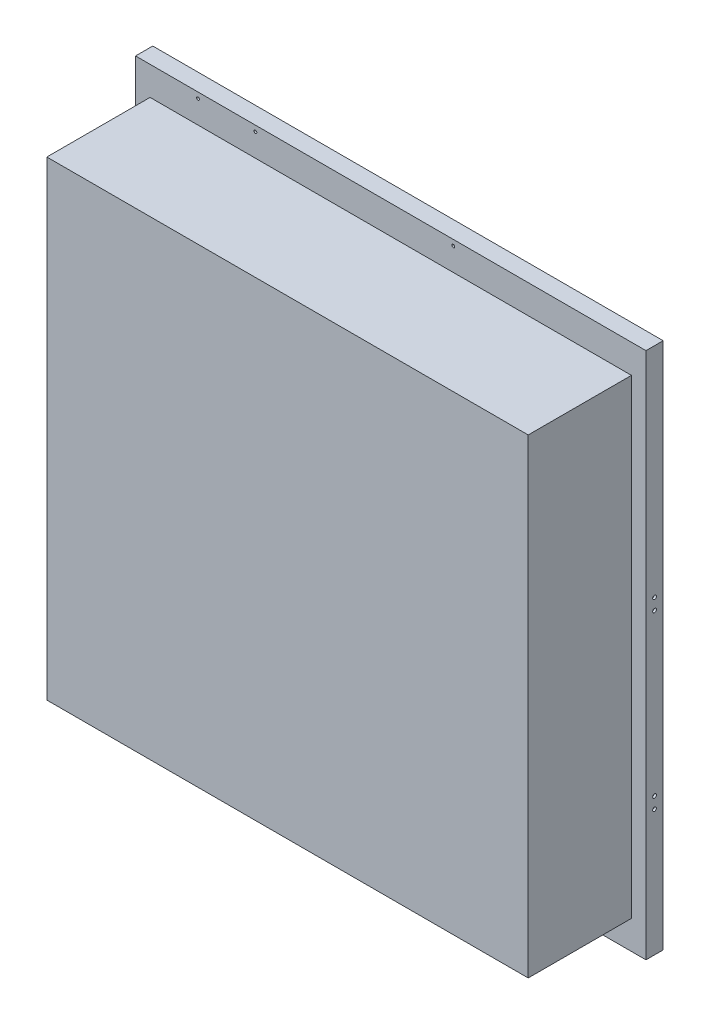
SolidWorks part; units mm, degrees
material "渡锌板"
ref_plane "前视基准面" through (0, 0, 0) normal (0, 0, 1) x (1, 0, 0)
ref_plane "上视基准面" through (0, 0, 0) normal (0, 1, 0) x (1, 0, 0)
ref_plane "右视基准面" through (0, 0, 0) normal (1, 0, 0) x (0, 0, -1)
sketch "草图1" plane through (0, 0, 0) normal (0, 0, 1) x (1, 0, 0)
  line L1 (-222.5, -235) -> (222.5, -235)
  line L2 (-222.5, -235) -> (-222.5, 235)
  line L3 (-222.5, 235) -> (222.5, 235)
  line L4 (222.5, -235) -> (222.5, 235)
  line L5 (-222.5, -235) -> (222.5, 235) construction
  line L6 (-222.5, 235) -> (222.5, -235) construction
  point P0 (0, 0)
  dimension "D1" = 445
  dimension "D2" = 470
extrude "凸台-拉伸1" add sketch "草图1" along normal mid plane 15
shell "抽壳1" thickness 2
sketch "草图2" plane through (0, 0, -7.5) normal (0, 0, -1) x (-1, 0, 0)
  line L0 (222.5, 235) -> (222.5, -235) construction
  line L1 (-212.5, -225) -> (212.5, -225)
  line L2 (-212.5, -225) -> (-212.5, 225)
  line L3 (-212.5, 225) -> (212.5, 225)
  line L4 (212.5, -225) -> (212.5, 225)
  line L5 (-212.5, -225) -> (212.5, 225) construction
  line L6 (-212.5, 225) -> (212.5, -225) construction
  line L7 (-222.5, 235) -> (222.5, 235) construction
  point P0 (0, 0)
  dimension "D1" = 10
  dimension "D2" = 10
extrude "切除-拉伸1" cut sketch "草图2" against normal blind 2
sketch "草图3" plane through (0, 0, 7.5) normal (0, 0, 1) x (1, 0, 0)
  line L0 (-205, 150) -> (-195, 150) construction
  line L1 (-200, -150) -> (200, -150) construction
  line L2 (-200, -150) -> (-200, 150) construction
  line L3 (-200, 150) -> (200, 150) construction
  line L4 (200, -150) -> (200, 150) construction
  line L5 (-200, -150) -> (200, 150) construction
  line L6 (-200, 150) -> (200, -150) construction
  line L7 (-205, 152.5) -> (-195, 152.5)
  line L8 (-205, 147.5) -> (-195, 147.5)
  line L9 (0, 235) -> (0, -235) construction
  line L10 (222.5, 235) -> (-222.5, 235) construction
  line L11 (-222.5, -235) -> (222.5, -235) construction
  line L12 (-222.5, 0) -> (222.5, 0) construction
  line L13 (-222.5, 235) -> (-222.5, -235) construction
  line L14 (222.5, -235) -> (222.5, 235) construction
  line L15 (195, 150) -> (205, 150) construction
  line L16 (195, 152.5) -> (205, 152.5)
  line L17 (195, 147.5) -> (205, 147.5)
  line L18 (-205, -150) -> (-195, -150) construction
  line L19 (-205, -147.5) -> (-195, -147.5)
  line L20 (-205, -152.5) -> (-195, -152.5)
  line L21 (195, -150) -> (205, -150) construction
  line L22 (195, -147.5) -> (205, -147.5)
  line L23 (195, -152.5) -> (205, -152.5)
  arc A0 (-205, 152.5) -> (-205, 147.5) centre (-205, 150) ccw
  arc A1 (-195, 147.5) -> (-195, 152.5) centre (-195, 150) ccw
  arc A2 (195, 152.5) -> (195, 147.5) centre (195, 150) ccw
  arc A3 (205, 147.5) -> (205, 152.5) centre (205, 150) ccw
  arc A4 (-205, -147.5) -> (-205, -152.5) centre (-205, -150) ccw
  arc A5 (-195, -152.5) -> (-195, -147.5) centre (-195, -150) ccw
  arc A6 (195, -147.5) -> (195, -152.5) centre (195, -150) ccw
  arc A7 (205, -152.5) -> (205, -147.5) centre (205, -150) ccw
  point P0 (0, 0)
  point P8 (-200, 150)
  point P27 (200, 150)
  point P34 (-200, -150)
  point P41 (200, -150)
  dimension "D4" = 2.5
  dimension "D6" = 2.5
  dimension "D8" = 2.5
  dimension "D9" = 2.5
  dimension "D1" = 400
  dimension "D2" = 300
  dimension "D3" = 10
  dimension "D5" = 10
  dimension "D7" = 10
  dimension "D10" = 10
extrude "切除-拉伸2" cut sketch "草图3" against normal blind 10
sketch "草图4" plane through (0, 0, 7.5) normal (0, 0, 1) x (1, 0, 0)
  line L0 (-222.5, -235) -> (222.5, -235) construction
  line L2 (222.5, -235) -> (222.5, 235) construction
  line B0 (147.5, -212.75) -> (147.5, -217.25) construction
  line B1 (37.5, -212.75) -> (37.5, -217.25) construction
  line B2 (-72.5, -212.75) -> (-72.5, -217.25) construction
  line B3 (164.75, 68) -> (159.2455, 68) construction
  line B4 (164.75, -25) -> (159.4595, -25) construction
  line B5 (147.5, -62.75) -> (147.5, -67.25) construction
  line B6 (37.5, -62.75) -> (37.5, -67.25) construction
  line B7 (-72.5, -62.75) -> (-72.5, -67.25) construction
  line B8 (-180.25, -65) -> (-184.75, -65) construction
  line B9 (-182.5, -62.75) -> (-182.5, -67.25) construction
  line B10 (17.25, -24) -> (11.5, -24) construction
  line B11 (15, -21.75) -> (15, -26.25) construction
  line B12 (-86.5, -21.75) -> (-86.5, -26.25) construction
  line B13 (1.75, 168.5) -> (-2.75, 168.5) construction
  line B14 (-0.5, 170.75) -> (-0.5, 166.25) construction
  line B15 (102.75, 129) -> (98.25, 129) construction
  line B16 (100.5, 131.25) -> (100.5, 126.75) construction
  line B17 (56.75, 225) -> (52.25, 225) construction
  line B18 (56.75, 177) -> (52.25, 177) construction
  line B19 (-172.5, -212.75) -> (-172.5, -217.25) construction
  line B20 (195.25, 72.4966) -> (190.75, 72.4966) construction
  line B21 (195.25, -202.5) -> (190.75, -202.5) construction
  line B22 (195.25, -92.5) -> (190.75, -92.5) construction
  line B23 (195.25, 17.5) -> (190.75, 17.5) construction
  line B24 (195.25, 7.5) -> (190.75, 7.5) construction
  line B25 (195.25, 202.4966) -> (190.75, 202.4966) construction
  line B26 (-175.75, 225) -> (-180.25, 225) construction
  line B27 (-83, -24) -> (-88.9344, -24) construction
  line B28 (47.25, -22.5) -> (51.75, -22.5) construction
  line B29 (47.25, 70.5) -> (51.75, 70.5) construction
  line B30 (222.5, -235) -> (-227.5, -235) construction
  line B31 (-227.5, -235) -> (-227.5, 235) construction
  line B32 (-227.5, 235) -> (222.5, 235) construction
  line B33 (222.5, 235) -> (222.5, -235) construction
  line B34 (-200, -152.5) -> (-205, -152.5) construction
  line B35 (-205, -147.5) -> (-200, -147.5) construction
  line B36 (200, 147.5) -> (195, 147.5) construction
  line B37 (195, 152.5) -> (200, 152.5) construction
  line B38 (200, -152.5) -> (195, -152.5) construction
  line B39 (195, -147.5) -> (200, -147.5) construction
  line B40 (-200, 147.5) -> (-205, 147.5) construction
  line B41 (-205, 152.5) -> (-200, 152.5) construction
  line B42 (145.25, -103.5) -> (149.75, -103.5) construction
  line B43 (145.25, -166.5) -> (149.75, -166.5) construction
  line B44 (71.5, -132.75) -> (71.5, -137.25) construction
  line B45 (-88.5, -132.75) -> (-88.5, -137.25) construction
  line B46 (-86.25, -135) -> (-90.75, -135) construction
  line B47 (-168.5, -132.75) -> (-168.5, -137.25) construction
  line B48 (-43.5, -132.75) -> (-43.5, -137.25) construction
  line B49 (-41.25, -135) -> (-45.75, -135) construction
  arc B50 (152.5, 186.5) -> (154, 185) centre (152.5, 185) ccw
  circle B51 centre (152.5, 185) radius 1.3
  arc B52 (152.5, 88.5) -> (154, 87) centre (152.5, 87) ccw
  circle B53 centre (152.5, 87) radius 1.3
  arc B54 (147.5, -213.5) -> (149, -215) centre (147.5, -215) ccw
  circle B55 centre (147.5, -215) radius 1.3
  arc B56 (37.5, -213.5) -> (39, -215) centre (37.5, -215) ccw
  circle B57 centre (37.5, -215) radius 1.3
  arc B58 (-72.5, -213.5) -> (-71, -215) centre (-72.5, -215) ccw
  circle B59 centre (-72.5, -215) radius 1.3
  arc B60 (162.5, 69.5) -> (164, 68) centre (162.5, 68) ccw
  circle B61 centre (162.5, 68) radius 1.3
  arc B62 (162.5, -23.5) -> (164, -25) centre (162.5, -25) ccw
  circle B63 centre (162.5, -25) radius 1.3
  arc B64 (147.5, -63.5) -> (149, -65) centre (147.5, -65) ccw
  circle B65 centre (147.5, -65) radius 1.3
  arc B66 (37.5, -63.5) -> (39, -65) centre (37.5, -65) ccw
  circle B67 centre (37.5, -65) radius 1.3
  arc B68 (-72.5, -63.5) -> (-71, -65) centre (-72.5, -65) ccw
  circle B69 centre (-72.5, -65) radius 1.3
  arc B70 (-182.5, -63.5) -> (-181, -65) centre (-182.5, -65) ccw
  circle B71 centre (-182.5, -65) radius 1.3
  arc B72 (15, -22.5) -> (16.5, -24) centre (15, -24) ccw
  circle B73 centre (15, -24) radius 1.3
  arc B74 (-86.5, -22.5) -> (-85, -24) centre (-86.5, -24) ccw
  circle B75 centre (-86.5, -24) radius 1.3
  arc B76 (-0.5, 170) -> (1, 168.5) centre (-0.5, 168.5) ccw
  circle B77 centre (-0.5, 168.5) radius 1.3
  arc B78 (100.5, 130.5) -> (102, 129) centre (100.5, 129) ccw
  circle B79 centre (100.5, 129) radius 1.3
  arc B80 (-178, -13.5) -> (-176.5, -15) centre (-178, -15) ccw
  circle B81 centre (-178, -15) radius 1.3
  arc B82 (-128, -13.5) -> (-126.5, -15) centre (-128, -15) ccw
  circle B83 centre (-128, -15) radius 1.3
  arc B84 (54.5, 226.5) -> (56, 225) centre (54.5, 225) ccw
  circle B85 centre (54.5, 225) radius 1.3
  arc B86 (54.5, 178.5) -> (56, 177) centre (54.5, 177) ccw
  circle B87 centre (54.5, 177) radius 1.3
  arc B88 (-172.5, -213.5) -> (-171, -215) centre (-172.5, -215) ccw
  circle B89 centre (-172.5, -215) radius 1.3
  arc B90 (193, 73.9966) -> (194.5, 72.4966) centre (193, 72.4966) ccw
  circle B91 centre (193, 72.4966) radius 1.3
  arc B92 (193, -201) -> (194.5, -202.5) centre (193, -202.5) ccw
  circle B93 centre (193, -202.5) radius 1.3
  arc B94 (193, -91) -> (194.5, -92.5) centre (193, -92.5) ccw
  circle B95 centre (193, -92.5) radius 1.3
  arc B96 (193, 19) -> (194.5, 17.5) centre (193, 17.5) ccw
  circle B97 centre (193, 17.5) radius 1.3
  arc B98 (194.5, 7.5) -> (193, 6) centre (193, 7.5) ccw
  circle B99 centre (193, 7.5) radius 1.3
  arc B100 (193, 203.9966) -> (194.5, 202.4966) centre (193, 202.4966) ccw
  circle B101 centre (193, 202.4966) radius 1.3
  arc B102 (-178, 226.5) -> (-176.5, 225) centre (-178, 225) ccw
  circle B103 centre (-178, 225) radius 1.3
  arc B104 (-128, 226.5) -> (-126.5, 225) centre (-128, 225) ccw
  circle B105 centre (-128, 225) radius 1.3
  arc B106 (134.5, 186.5) -> (136, 185) centre (134.5, 185) ccw
  circle B107 centre (134.5, 185) radius 1.3
  arc B108 (134.5, 88.5) -> (136, 87) centre (134.5, 87) ccw
  circle B109 centre (134.5, 87) radius 1.3
  arc B110 (48, -22.5) -> (49.5, -21) centre (49.5, -22.5) ccw
  circle B111 centre (49.5, -22.5) radius 1.3
  arc B112 (48, 70.5) -> (49.5, 72) centre (49.5, 70.5) ccw
  circle B113 centre (49.5, 70.5) radius 1.3
  arc B114 (-205, -147.5) -> (-205, -152.5) centre (-205, -150) ccw construction
  arc B115 (-200, -152.5) -> (-200, -147.5) centre (-200, -150) ccw construction
  arc B116 (195, 152.5) -> (195, 147.5) centre (195, 150) ccw construction
  arc B117 (200, 147.5) -> (200, 152.5) centre (200, 150) ccw construction
  arc B118 (195, -147.5) -> (195, -152.5) centre (195, -150) ccw construction
  arc B119 (200, -152.5) -> (200, -147.5) centre (200, -150) ccw construction
  arc B120 (-205, 152.5) -> (-205, 147.5) centre (-205, 150) ccw construction
  arc B121 (-200, 147.5) -> (-200, 152.5) centre (-200, 150) ccw construction
  arc B122 (146, -103.5) -> (147.5, -102) centre (147.5, -103.5) ccw
  circle B123 centre (147.5, -103.5) radius 1.3
  arc B124 (146, -166.5) -> (147.5, -165) centre (147.5, -166.5) ccw
  circle B125 centre (147.5, -166.5) radius 1.3
  arc B126 (71.5, -133.5) -> (73, -135) centre (71.5, -135) ccw
  circle B127 centre (71.5, -135) radius 1.3
  arc B128 (-88.5, -133.5) -> (-87, -135) centre (-88.5, -135) ccw
  circle B129 centre (-88.5, -135) radius 1.3
  arc B130 (-168.5, -133.5) -> (-167, -135) centre (-168.5, -135) ccw
  circle B131 centre (-168.5, -135) radius 1.3
  arc B132 (-43.5, -133.5) -> (-42, -135) centre (-43.5, -135) ccw
  circle B133 centre (-43.5, -135) radius 1.3
sketch_block_instance "块1-1"
sketch_block "块1" parameters "D1"=1.5
hole_wizard "M3 螺纹孔1" positions "草图6" profile "草图5" tap size "M3" standard "GB"
sketch "草图6" plane through (0, 0, 7.5) normal (0, 0, 1) x (1, 0, 0)
  line L0 (222.5, 235) -> (-222.5, 235) construction
  line L1 (222.5, -235) -> (222.5, 235) construction
  line L2 (-222.5, 235) -> (-222.5, -235) construction
  line L3 (-222.5, -235) -> (222.5, -235) construction
  line L4 (-222.5, 235) -> (-222.5, -235) construction
  point P1 (-72.5, -215)
  point P4 (-172.5, -215)
  point P7 (37.5, -215)
  point P10 (147.5, -215)
  point P13 (193, -202.5)
  point P16 (147.5, -166.5)
  point P19 (66.5, -135)
  point P22 (-13.5, -135)
  point P25 (-58.5, -135)
  point P28 (-173.5, -135)
  point P31 (-182.5, -65)
  point P34 (-168, -15)
  point P37 (-118, -15)
  point P40 (-72.5, -65)
  point P43 (-81.5, -24)
  point P46 (37.5, -65)
  point P49 (15, -24)
  point P52 (49.5, -22.5)
  point P55 (147.5, -103.5)
  point P58 (193, -92.5)
  point P61 (147.5, -65)
  point P64 (162.5, -25)
  point P67 (193, 7.5)
  point P70 (193, 17.5)
  point P73 (193, 72.4966)
  point P76 (162.5, 68)
  point P79 (152.5, 27)
  point P82 (134.5, 27)
  point P85 (100.5, 129)
  point P88 (49.5, 70.5)
  point P91 (193, 202.4966)
  point P94 (152.5, 125)
  point P97 (134.5, 125)
  point P100 (54.5, 177)
  point P103 (54.5, 225)
  point P106 (4.5, 168.5)
  point P109 (-118, 225)
  point P112 (-168, 225)
  point P155 (-222.5, 0)
  dimension "D1" = 98
  dimension "D2" = 18
  dimension "D3" = 110
  dimension "D4" = 70
  dimension "D5" = 49
  dimension "D6" = 115
  dimension "D7" = 45
  dimension "D8" = 80
  dimension "D9" = 100
  dimension "D10" = 50
  dimension "D11" = 240
  dimension "D12" = 10
  dimension "D13" = 54.5
  dimension "D14" = 141
  dimension "D15" = 259
  dimension "D16" = 227
  dimension "D17" = 66.5
sketch "草图5" plane through (-72.5, -215, 7.5) normal (1, 0, 0) x (0, -1, 0)
  line L0 (0, 0) -> (0, 7.5)
  line L1 (0, 7.5) -> (1.25, 7.5)
  line L2 (1.25, 7.5) -> (1.25, 0)
  line L5 (1.25, 0) -> (0, 0)
  line L10 (0, 7.5) -> (-1.25, 7.5) construction
  line L11 (0, -6.35) -> (0, 107.95) construction
  dimension "螺纹孔钻头直径" = 2.5
  dimension "螺纹孔钻头深度" = 7.5
  dimension "导头角度" = 180
cosmetic thread "孔螺蚊线1" parameters "D1"=1.5, "D2"=3
cosmetic thread "孔螺蚊线2" parameters "D1"=1.5, "D2"=3
cosmetic thread "孔螺蚊线3" parameters "D1"=1.5, "D2"=3
cosmetic thread "孔螺蚊线4" parameters "D1"=1.5, "D2"=3
cosmetic thread "孔螺蚊线5" parameters "D1"=1.5, "D2"=3
cosmetic thread "孔螺蚊线6" parameters "D1"=1.5, "D2"=3
cosmetic thread "孔螺蚊线7" parameters "D1"=1.5, "D2"=3
cosmetic thread "孔螺蚊线8" parameters "D1"=1.5, "D2"=3
cosmetic thread "孔螺蚊线9" parameters "D1"=1.5, "D2"=3
cosmetic thread "孔螺蚊线10" parameters "D1"=1.5, "D2"=3
cosmetic thread "孔螺蚊线11" parameters "D1"=1.5, "D2"=3
cosmetic thread "孔螺蚊线12" parameters "D1"=1.5, "D2"=3
cosmetic thread "孔螺蚊线13" parameters "D1"=1.5, "D2"=3
cosmetic thread "孔螺蚊线14" parameters "D1"=1.5, "D2"=3
cosmetic thread "孔螺蚊线15" parameters "D1"=1.5, "D2"=3
cosmetic thread "孔螺蚊线16" parameters "D1"=1.5, "D2"=3
cosmetic thread "孔螺蚊线17" parameters "D1"=1.5, "D2"=3
cosmetic thread "孔螺蚊线18" parameters "D1"=1.5, "D2"=3
cosmetic thread "孔螺蚊线19" parameters "D1"=1.5, "D2"=3
cosmetic thread "孔螺蚊线20" parameters "D1"=1.5, "D2"=3
cosmetic thread "孔螺蚊线21" parameters "D1"=1.5, "D2"=3
cosmetic thread "孔螺蚊线22" parameters "D1"=1.5, "D2"=3
cosmetic thread "孔螺蚊线23" parameters "D1"=1.5, "D2"=3
cosmetic thread "孔螺蚊线24" parameters "D1"=1.5, "D2"=3
cosmetic thread "孔螺蚊线25" parameters "D1"=1.5, "D2"=3
cosmetic thread "孔螺蚊线26" parameters "D1"=1.5, "D2"=3
cosmetic thread "孔螺蚊线27" parameters "D1"=1.5, "D2"=3
cosmetic thread "孔螺蚊线28" parameters "D1"=1.5, "D2"=3
cosmetic thread "孔螺蚊线29" parameters "D1"=1.5, "D2"=3
cosmetic thread "孔螺蚊线30" parameters "D1"=1.5, "D2"=3
cosmetic thread "孔螺蚊线31" parameters "D1"=1.5, "D2"=3
cosmetic thread "孔螺蚊线32" parameters "D1"=1.5, "D2"=3
cosmetic thread "孔螺蚊线33" parameters "D1"=1.5, "D2"=3
cosmetic thread "孔螺蚊线34" parameters "D1"=1.5, "D2"=3
cosmetic thread "孔螺蚊线35" parameters "D1"=1.5, "D2"=3
cosmetic thread "孔螺蚊线36" parameters "D1"=1.5, "D2"=3
cosmetic thread "孔螺蚊线37" parameters "D1"=1.5, "D2"=3
cosmetic thread "孔螺蚊线38" parameters "D1"=1.5, "D2"=3
sketch "草图7" plane through (0, 235, 0) normal (0, 1, 0) x (1, 0, 0)
  line L0 (222.5, -7.5) -> (222.5, 7.5) construction
  line L1 (-222.5, 7.5) -> (222.5, 7.5)
  line L2 (-222.5, 7.5) -> (-222.5, -6)
  line L3 (-222.5, -6) -> (222.5, -6)
  line L4 (222.5, 7.5) -> (222.5, -6)
  line L5 (222.5, -7.5) -> (-222.5, -7.5) construction
  dimension "D1" = 1.5
extrude "切除-拉伸3" [suppressed] cut sketch "草图7" against normal through all
sketch "草图9" plane through (0, 0, 7.5) normal (0, 0, 1) x (1, 0, 0)
  line L0 (222.5, -235) -> (222.5, 235) construction
  line L1 (-222.5, 235) -> (222.5, 235)
  line L2 (-222.5, 235) -> (-222.5, 230)
  line L3 (-222.5, 230) -> (222.5, 230)
  line L4 (222.5, 235) -> (222.5, 230)
  line L6 (-222.5, -235) -> (222.5, -235)
  line L7 (-222.5, -235) -> (-222.5, -230)
  line L8 (-222.5, -230) -> (222.5, -230)
  line L9 (222.5, -235) -> (222.5, -230)
  dimension "D1" = 5
  dimension "D2" = 5
extrude "切除-拉伸4" cut sketch "草图9" against normal through all
sketch "草图10" plane through (0, 230, 0) normal (0, 1, 0) x (1, 0, 0)
  line L4 (-222.5, -7.5) -> (222.5, -7.5)
  line L5 (222.5, -7.5) -> (222.5, 7.5)
  line L6 (222.5, 7.5) -> (-222.5, 7.5)
  line L7 (-222.5, 7.5) -> (-222.5, -7.5)
  line L8 (-222.5, -7.5) -> (222.5, -7.5)
  line L9 (222.5, -7.5) -> (222.5, 7.5)
  line L10 (222.5, 7.5) -> (-222.5, 7.5)
  line L11 (-222.5, 7.5) -> (-222.5, -7.5)
  dimension "D1" = 0
extrude "凸台-拉伸2" add sketch "草图10" against normal blind 1.5
sketch "草图11" plane through (0, -230, 0) normal (0, -1, 0) x (1, 0, 0)
  line L4 (222.5, 7.5) -> (-222.5, 7.5)
  line L5 (-222.5, 7.5) -> (-222.5, -7.5)
  line L6 (-222.5, -7.5) -> (222.5, -7.5)
  line L7 (222.5, -7.5) -> (222.5, 7.5)
  line L8 (222.5, 7.5) -> (-222.5, 7.5)
  line L9 (-222.5, 7.5) -> (-222.5, -7.5)
  line L10 (-222.5, -7.5) -> (222.5, -7.5)
  line L11 (222.5, -7.5) -> (222.5, 7.5)
  dimension "D1" = 0
extrude "凸台-拉伸3" add sketch "草图11" against normal blind 1.5
other "移动面1" face at (0, 225, -6.5) parameters "D1"=5
other "移动面2" face at (0, -225, -6.5) parameters "D1"=5
sketch "草图12" plane through (0, 0, 7.5) normal (0, 0, 1) x (1, 0, 0)
  line L0 (-195, 152.5) -> (-205, 152.5) construction
  line L1 (-205, 147.5) -> (-195, 147.5) construction
  line L2 (-195, 152.5) -> (-205, 152.5)
  line L3 (-205, 147.5) -> (-195, 147.5)
  line L4 (-195, -147.5) -> (-205, -147.5) construction
  line L5 (-205, -152.5) -> (-195, -152.5) construction
  line L6 (-195, -147.5) -> (-205, -147.5)
  line L7 (-205, -152.5) -> (-195, -152.5)
  line L8 (205, 152.5) -> (195, 152.5) construction
  line L9 (195, 147.5) -> (205, 147.5) construction
  line L10 (205, 152.5) -> (195, 152.5)
  line L11 (195, 147.5) -> (205, 147.5)
  line L12 (205, -147.5) -> (195, -147.5) construction
  line L13 (195, -152.5) -> (205, -152.5) construction
  line L14 (205, -147.5) -> (195, -147.5)
  line L15 (195, -152.5) -> (205, -152.5)
  arc A0 (-205, 152.5) -> (-205, 147.5) centre (-205, 150) ccw construction
  arc A1 (-195, 147.5) -> (-195, 152.5) centre (-195, 150) ccw construction
  arc A2 (-205, 152.5) -> (-205, 147.5) centre (-205, 150) ccw
  arc A3 (-195, 147.5) -> (-195, 152.5) centre (-195, 150) ccw
  arc A4 (-205, -147.5) -> (-205, -152.5) centre (-205, -150) ccw construction
  arc A5 (-195, -152.5) -> (-195, -147.5) centre (-195, -150) ccw construction
  arc A6 (-205, -147.5) -> (-205, -152.5) centre (-205, -150) ccw
  arc A7 (-195, -152.5) -> (-195, -147.5) centre (-195, -150) ccw
  arc A8 (195, 152.5) -> (195, 147.5) centre (195, 150) ccw construction
  arc A9 (205, 147.5) -> (205, 152.5) centre (205, 150) ccw construction
  arc A10 (195, 152.5) -> (195, 147.5) centre (195, 150) ccw
  arc A11 (205, 147.5) -> (205, 152.5) centre (205, 150) ccw
  arc A12 (195, -147.5) -> (195, -152.5) centre (195, -150) ccw construction
  arc A13 (205, -152.5) -> (205, -147.5) centre (205, -150) ccw construction
  arc A14 (195, -147.5) -> (195, -152.5) centre (195, -150) ccw
  arc A15 (205, -152.5) -> (205, -147.5) centre (205, -150) ccw
extrude "凸台-拉伸4" add sketch "草图12" against normal up to surface (2 mm away) up to face at (-73.75, -215, 5.5)
sketch "草图13" plane through (0, 0, -7.5) normal (0, 0, -1) x (-1, 0, 0)
  line L1 (-217.8338, -48.6163) -> (-214.6504, -48.6163)
  line L2 (-217.8338, -48.6163) -> (-217.8338, -42.5242)
  line L3 (-217.8338, -42.5242) -> (-214.6504, -42.5242)
  line L4 (-214.6504, -48.6163) -> (-214.6504, -42.5242)
  line L5 (-217.8338, -48.6163) -> (-214.6504, -42.5242) construction
  line L6 (-217.8338, -42.5242) -> (-214.6504, -48.6163) construction
  point P0 (-216.2421, -45.5702)
sketch "草图14" plane through (0, 0, -7.5) normal (0, 0, -1) x (-1, 0, 0)
  line L0 (-212.5, 220) -> (-212.5, -220) construction
  line L1 (-212.5, 180) -> (-220.5, 180)
  line L2 (-212.5, 180) -> (-212.5, -180)
  line L3 (-212.5, -180) -> (-220.5, -180)
  line L4 (-220.5, 180) -> (-220.5, -180)
  line L5 (0, 230) -> (0, -230) construction
  line L6 (222.5, 230) -> (-222.5, 230) construction
  line L7 (-222.5, -230) -> (222.5, -230) construction
  line L8 (-222.5, -230) -> (-222.5, 230) construction
  line L9 (220.5, 180) -> (220.5, -180)
  line L10 (212.5, -180) -> (220.5, -180)
  line L11 (212.5, 180) -> (212.5, -180)
  line L12 (212.5, 180) -> (220.5, 180)
  dimension "D1" = 2
  dimension "D2" = 50
  dimension "D3" = 50
extrude "切除-拉伸6" [suppressed] cut sketch "草图14" against normal blind 2
fillet "圆角1" [suppressed] radius 3
hole_wizard "M4 螺纹孔1" positions "草图16" profile "草图17" tap size "M4" standard "GB" end condition through all
sketch "草图16" plane through (-222.5, 0, 0) normal (-1, 0, 0) x (0, 0, 1)
  line L0 (-7.5, 0) -> (7.5, 0) construction
  line L1 (-7.5, 230) -> (-7.5, -230) construction
  line L2 (7.5, 230) -> (7.5, -230) construction
  line L4 (-7.5, 230) -> (7.5, 230) construction
  line L5 (-7.5, -230) -> (7.5, -230) construction
  point P0 (0, 30)
  point P14 (0, -120)
  dimension "D1" = 7.5
  dimension "D2" = 200
  dimension "D3" = 110
sketch "草图17" plane through (-222.5, 30, 0) normal (0, 1, 0) x (0, 0, 1)
  line L0 (0, 0) -> (0, 445)
  line L1 (0, 445) -> (1.65, 445)
  line L2 (1.65, 445) -> (1.65, 0)
  line L5 (1.65, 0) -> (0, 0)
  line L11 (0, -6.35) -> (0, 107.95) construction
  dimension "通孔螺纹孔钻头直径" = 3.3
  dimension "通孔螺纹孔钻头深度" = 445
cosmetic thread "孔螺蚊线39" parameters "D2"=4
cosmetic thread "孔螺蚊线40" parameters "D2"=4
hole_wizard "M3 螺纹孔2" positions "草图21" profile "草图20" tap size "M3" standard "GB" end condition through all
sketch "草图21" plane through (0, 0, 7.5) normal (0, 0, 1) x (1, 0, 0)
  line L0 (-58.5, -135) -> (110, -135) construction
  point P0 (-43.5, -135)
  point P4 (110, -135)
  dimension "D1" = 15
  dimension "D2" = 153.5
sketch "草图20" plane through (-43.5, -135, 7.5) normal (1, 0, 0) x (0, -1, 0)
  line L0 (0, 0) -> (0, 15)
  line L1 (0, 15) -> (1.25, 15)
  line L2 (1.25, 15) -> (1.25, 0)
  line L5 (1.25, 0) -> (0, 0)
  line L11 (0, -6.35) -> (0, 107.95) construction
  dimension "通孔螺纹孔钻头直径" = 2.5
  dimension "通孔螺纹孔钻头深度" = 15
cosmetic thread "孔螺蚊线43" parameters "D2"=3
cosmetic thread "孔螺蚊线44" parameters "D2"=3
hole_wizard "M3 螺纹孔3" positions "草图23" profile "草图22" tap size "M3" standard "GB" end condition through all
sketch "草图23" plane through (0, 0, 7.5) normal (0, 0, 1) x (1, 0, 0)
  line L0 (15, -24) -> (-71, -24) construction
  line L1 (-71, -24) -> (-71, 167.5) construction
  point P0 (-71, 167.5)
  dimension "D1" = 86
  dimension "D2" = 191.5
sketch "草图22" plane through (-71, 167.5, 7.5) normal (1, 0, 0) x (0, -1, 0)
  line L0 (0, 0) -> (0, 15)
  line L1 (0, 15) -> (1.25, 15)
  line L2 (1.25, 15) -> (1.25, 0)
  line L5 (1.25, 0) -> (0, 0)
  line L11 (0, -6.35) -> (0, 107.95) construction
  dimension "通孔螺纹孔钻头直径" = 2.5
  dimension "通孔螺纹孔钻头深度" = 15
cosmetic thread "孔螺蚊线45" parameters "D2"=3
pattern_linear "阵列(线性)1" count 2 spacing 10 along (0, 1, 0) of "M4 螺纹孔1"
hole_wizard "M3 螺纹孔4" positions "草图25" profile "草图24" tap size "M3" standard "GB" end condition through all
sketch "草图25" plane through (0, 0, 7.5) normal (0, 0, 1) x (1, 0, 0)
  line L0 (-222.5, 230) -> (222.5, 230) construction
  line L1 (222.5, -230) -> (222.5, 230) construction
  point P0 (109.5, 187)
  point P2 (137.5, 187)
  point P9 (109.5, -5)
  point P11 (137.5, -5)
  dimension "D1" = 43
  dimension "D2" = 28
  dimension "D3" = 85
  dimension "D4" = 192
sketch "草图24" plane through (109.5, 187, 7.5) normal (1, 0, 0) x (0, -1, 0)
  line L0 (0, 0) -> (0, 15)
  line L1 (0, 15) -> (1.25, 15)
  line L2 (1.25, 15) -> (1.25, 0)
  line L5 (1.25, 0) -> (0, 0)
  line L11 (0, -6.35) -> (0, 107.95) construction
  dimension "通孔螺纹孔钻头直径" = 2.5
  dimension "通孔螺纹孔钻头深度" = 15
cosmetic thread "孔螺蚊线46" parameters "D2"=3
cosmetic thread "孔螺蚊线47" parameters "D2"=3
cosmetic thread "孔螺蚊线48" parameters "D2"=3
cosmetic thread "孔螺蚊线49" parameters "D2"=3
sketch "草图26" plane through (0, 0, 7.5) normal (0, 0, 1) x (1, 0, 0)
  line L1 (-209.842, 205.0174) -> (209.842, 205.0174)
  line L2 (-209.842, 205.0174) -> (-209.842, -205.0174)
  line L3 (-209.842, -205.0174) -> (209.842, -205.0174)
  line L4 (209.842, 205.0174) -> (209.842, -205.0174)
  line L5 (-209.842, 205.0174) -> (209.842, -205.0174) construction
  line L6 (-209.842, -205.0174) -> (209.842, 205.0174) construction
  point P0 (0, 0)
extrude "凸台-拉伸5" add sketch "草图26" along normal blind 90
